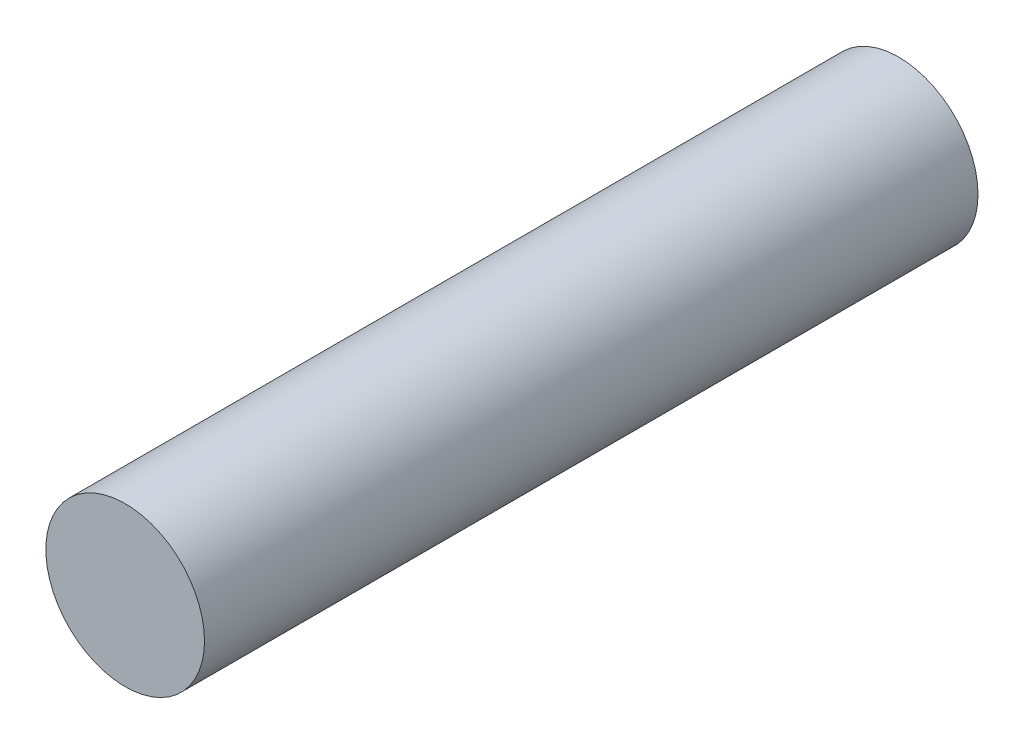
from build123d import *

# Parameters (mm, degrees)
SKETCH_1_R      = 4
EXTRUDE_1_DEPTH = 39


with BuildPart() as part:
    # 草图1 → 凸台-拉伸1 (new body)
    with BuildSketch(Plane.XY):
        Circle(SKETCH_1_R)
    extrude(amount=EXTRUDE_1_DEPTH)


solid = part.part
